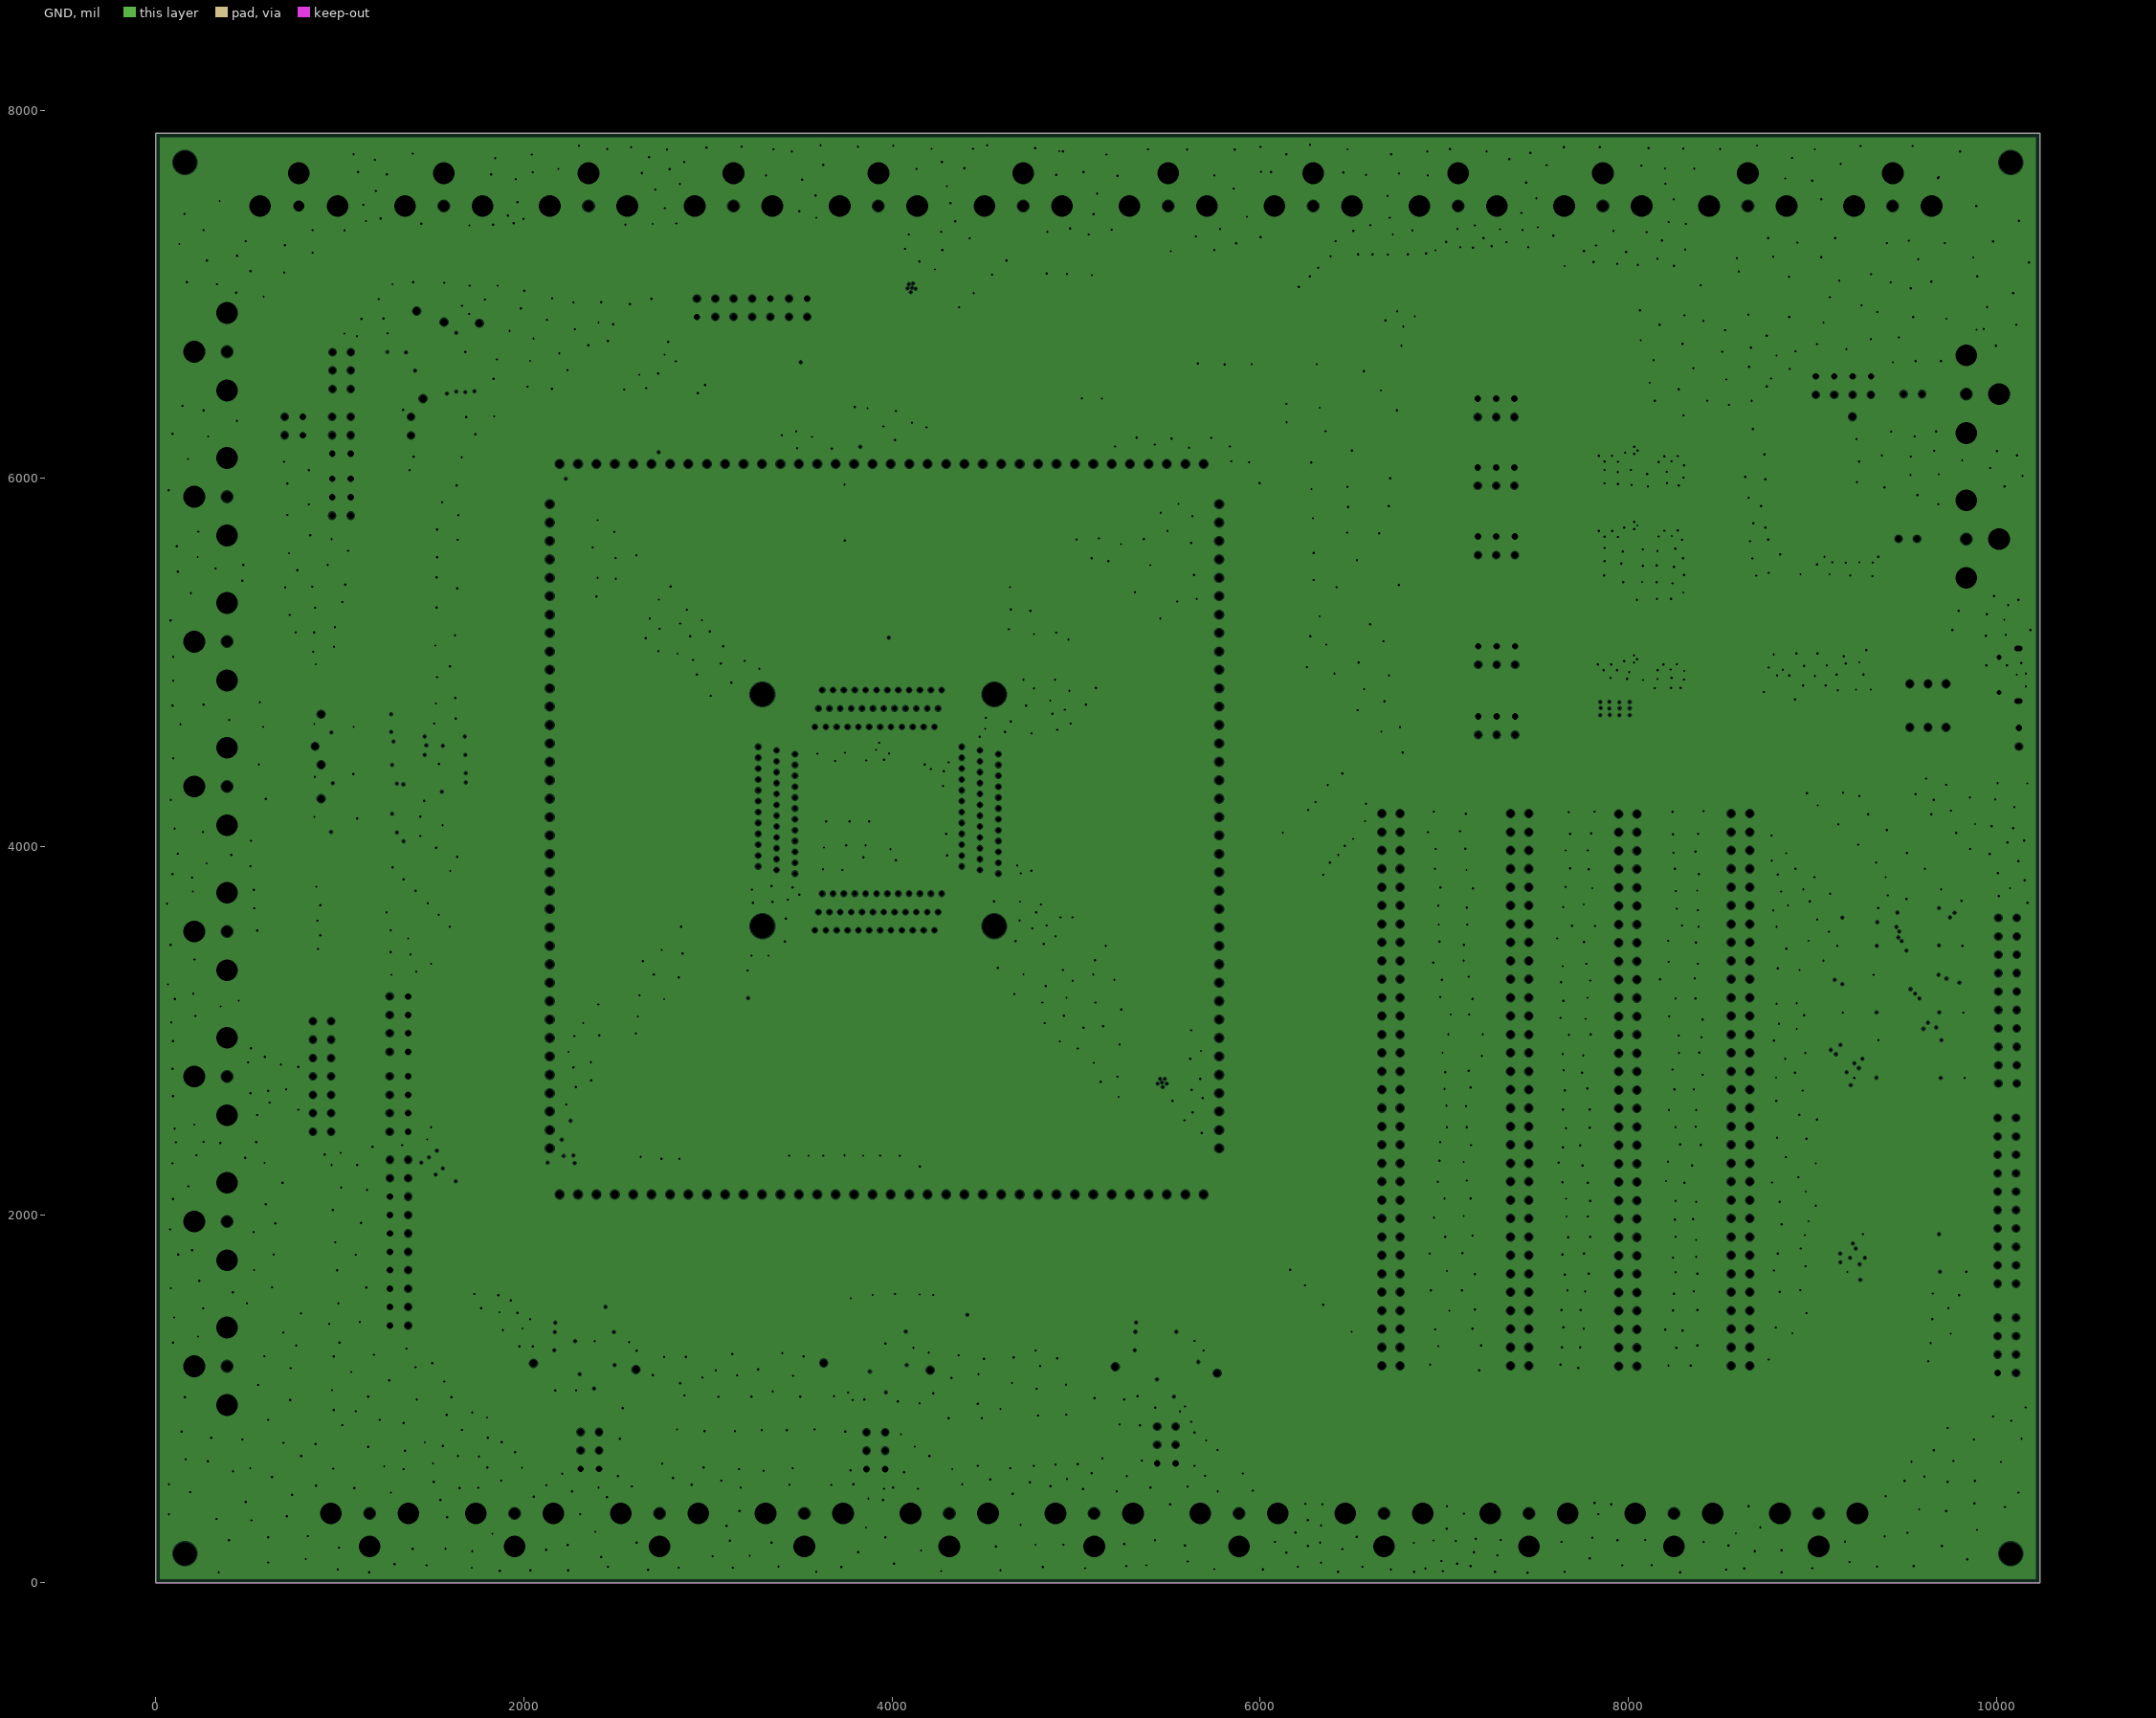
[diagram p0: GND, clearances drawn from the general rule]
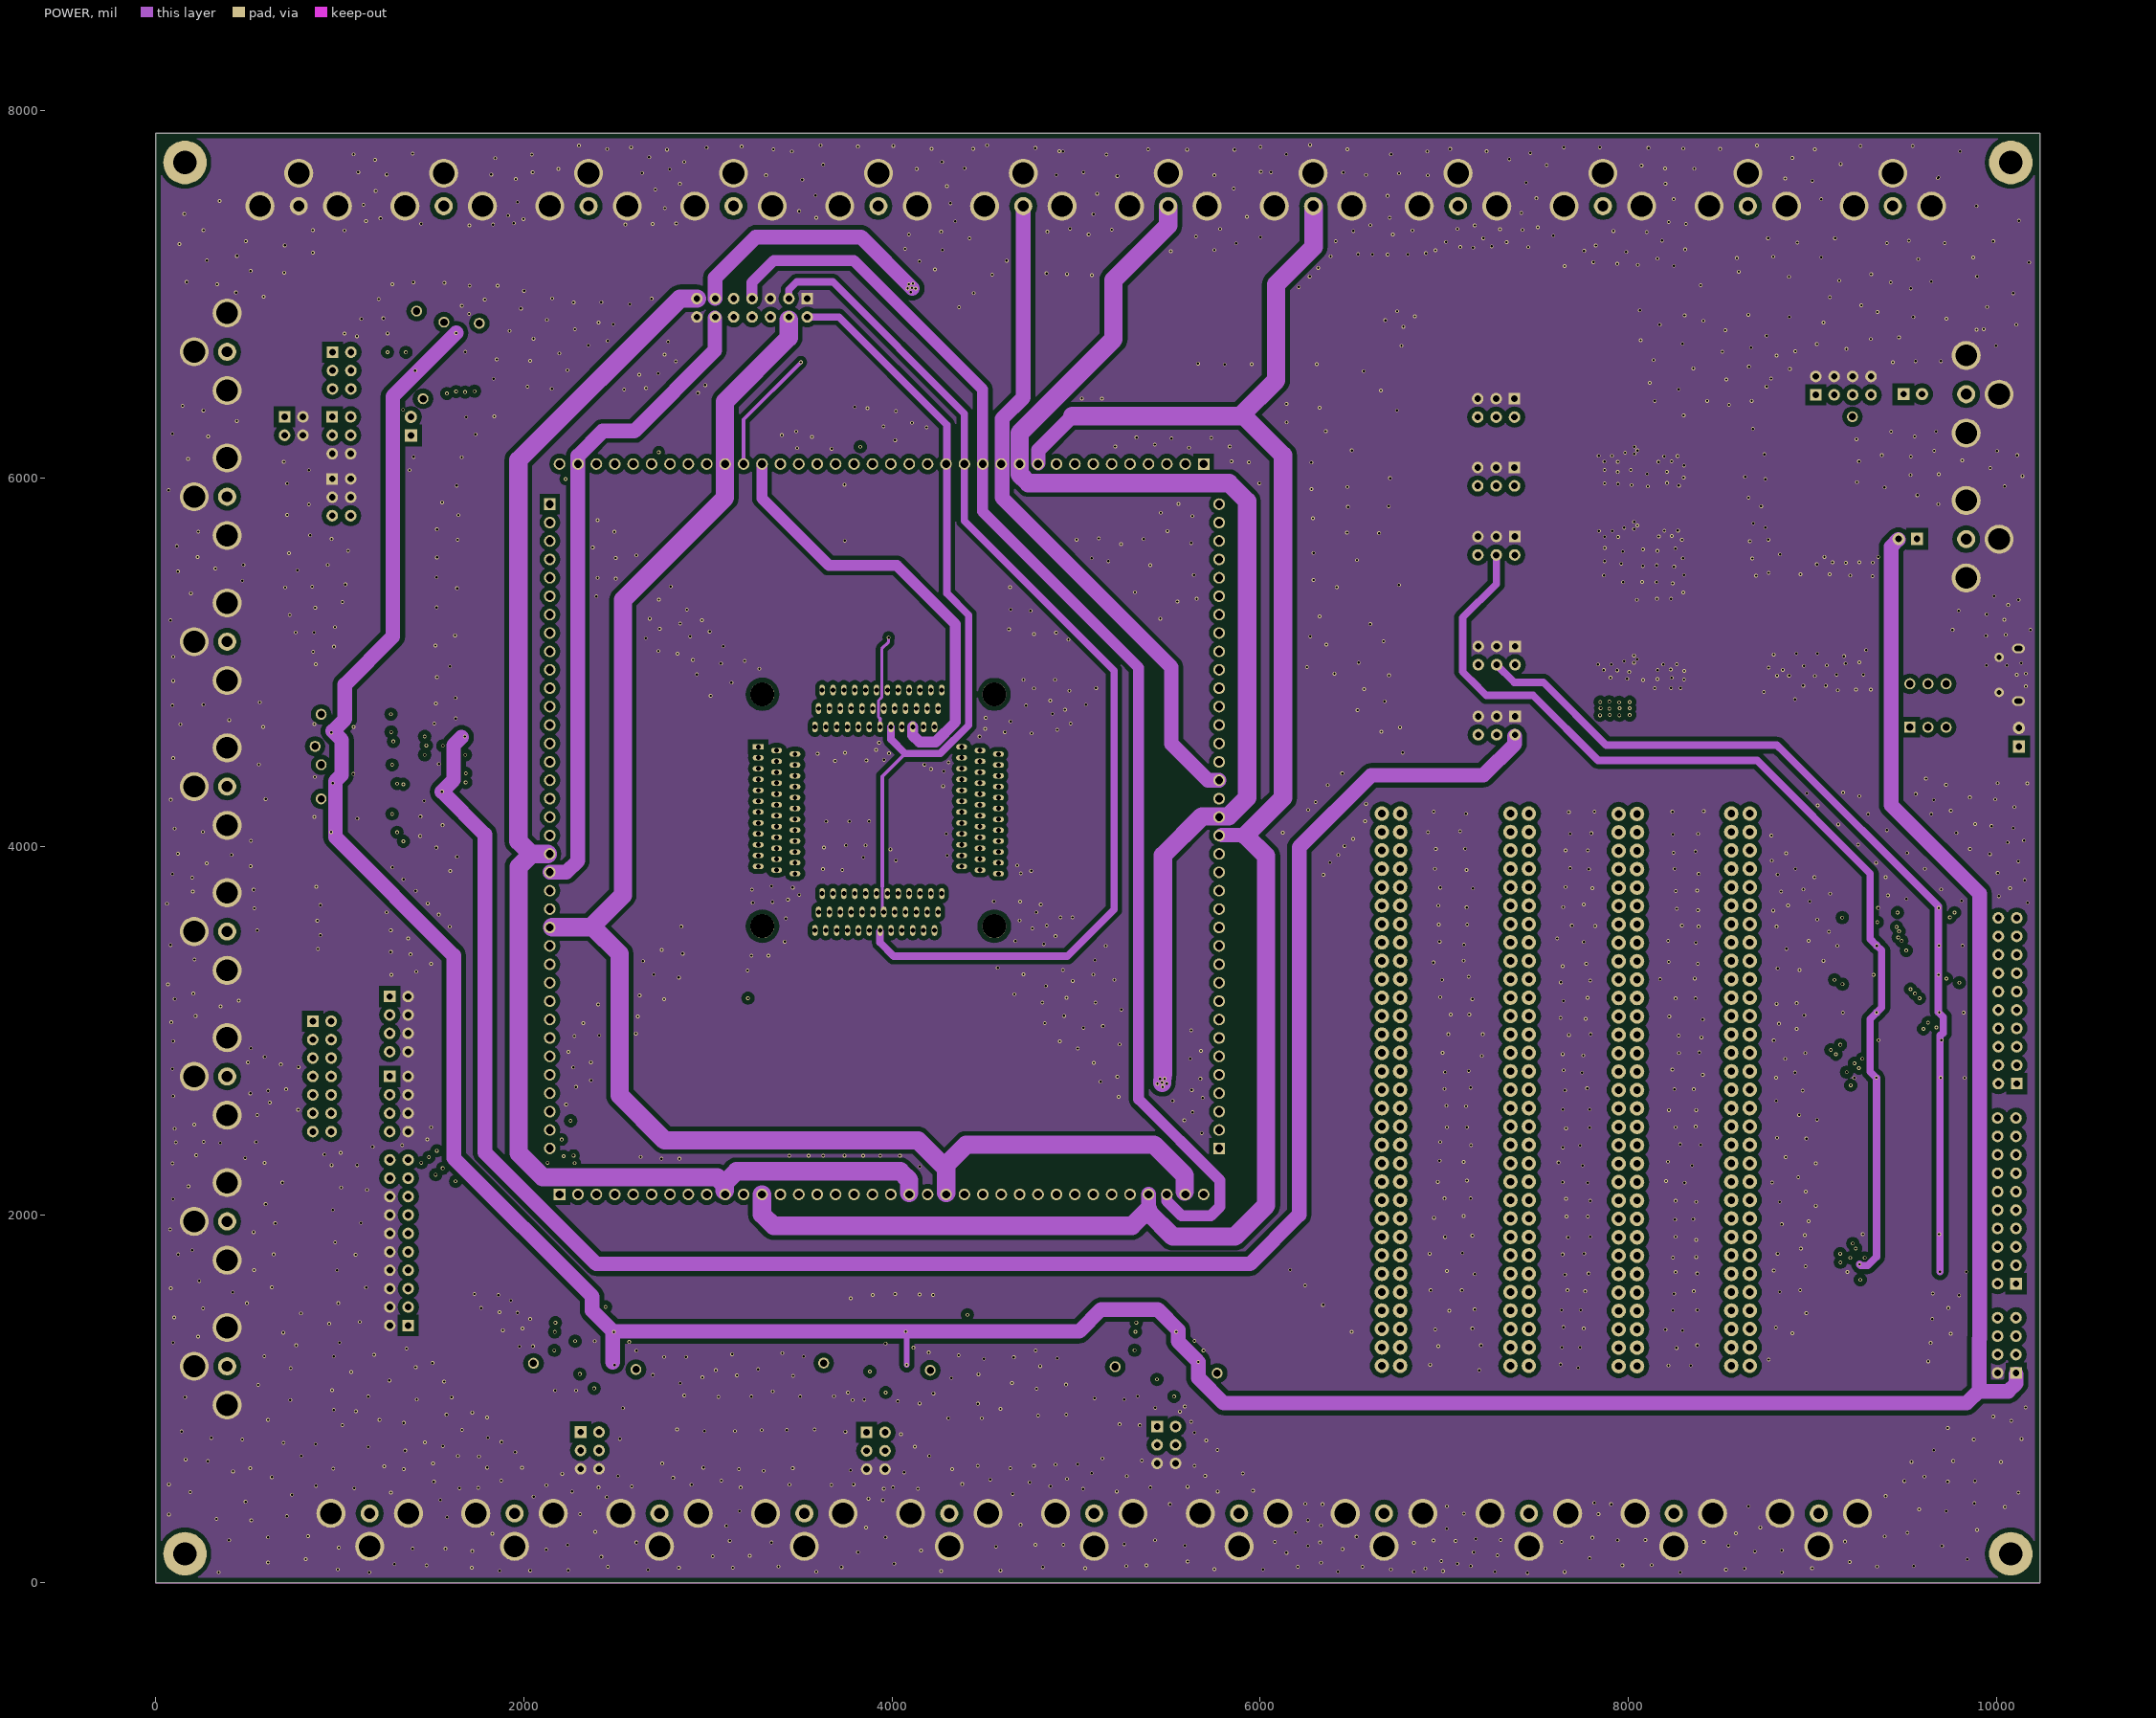
[diagram p1: POWER]
# Altium PCB MISC62794.PcbDoc (part 2 of 7)
## Footprints (in the part's own frame and the unit in brackets; to place one, negate y for a bottom-side part, rotate by r counter-clockwise, add the part's x,y. Pads: shape width x height; smd on the part's side, far side on the other; paste and mask are expansions set on the pad) (continued)
HDR2.54-LI-2x10P [mm] "双排排针，10x2脚"
  rect 1.6x1.6 hole 0.9: 1(-11.43,-1.27)
  round 1.6 hole 0.9: 2(-11.43,1.27) 3(-8.89,-1.27) 4(-8.89,1.27) 5(-6.35,-1.27) 6(-6.35,1.27) 7(-3.81,-1.27) 8(-3.81,1.27) 9(-1.27,-1.27) 10(-1.27,1.27) 11(1.27,-1.27) 12(1.27,1.27) 13(3.81,-1.27) 14(3.81,1.27) 15(6.35,-1.27) 16(6.35,1.27) 17(8.89,-1.27) 18(8.89,1.27) 19(11.43,-1.27) 20(11.43,1.27)
  silkscreen extent -12.7,-2.54 12.7,2.54, body extent -12.7,-2.54 12.7,2.54, height 8.5
HDR2.54-LI-2x31P [mm]
  round 2 hole 1.02: 1(-38.1,1.27) 2(-38.1,-1.27) 3(-35.56,1.27) 4(-35.56,-1.27) 5(-33.02,1.27) 6(-33.02,-1.27) 7(-30.48,1.27) 8(-30.48,-1.27) 9(-27.94,1.27) 10(-27.94,-1.27) 11(-25.4,1.27) 12(-25.4,-1.27) 13(-22.86,1.27) 14(-22.86,-1.27) 15(-20.32,1.27) 16(-20.32,-1.27) 17(-17.78,1.27) 18(-17.78,-1.27) 19(-15.24,1.27) 20(-15.24,-1.27) 21(-12.7,1.27) 22(-12.7,-1.27) 23(-10.16,1.27) 24(-10.16,-1.27) 25(-7.62,1.27) 26(-7.62,-1.27) 27(-5.08,1.27) 28(-5.08,-1.27) 29(-2.54,1.27) 30(-2.54,-1.27) 31(0,1.27) 32(0,-1.27) 33(2.54,1.27) 34(2.54,-1.27) 35(5.08,1.27) 36(5.08,-1.27) 37(7.62,1.27) 38(7.62,-1.27) 39(10.16,1.27) 40(10.16,-1.27) 41(12.7,1.27) 42(12.7,-1.27) 43(15.24,1.27) 44(15.24,-1.27) 45(17.78,1.27) 46(17.78,-1.27) 47(20.32,1.27) 48(20.32,-1.27) 49(22.86,1.27) 50(22.86,-1.27) 51(25.4,1.27) 52(25.4,-1.27) 53(27.94,1.27) 54(27.94,-1.27) 55(30.48,1.27) 56(30.48,-1.27) 57(33.02,1.27) 58(33.02,-1.27) 59(35.56,1.27) 60(35.56,-1.27) 61(38.1,1.27) 62(38.1,-1.27)
  silkscreen extent -39.4,-2.5 39.4,2.5
LED0805-R-RD [mm]
  rect 1x1.4 smd: 1(1.05,0) 2(-1.05,0)
  silkscreen extent -2.22,-1.04 1.99,1.01
M3 [mm]
  round 6 hole 3.2: 1(0,0)
MICRO-USB-SMD_MICROXNJ [mm]
  rect 0.4x1.6 smd paste-100 mask+0.051: 1(-1.3,2.619) 2(-0.65,2.619) 3(0,2.619) 4(0.65,2.619) 5(1.3,2.619)
  round 1.3 hole 0.7 paste+0 mask+0.051: 6(2.425,2.096) 9(-2.425,2.096)
  oval 1.3x1.8 hole 0.7 slot 1.1 at 90 deg paste+0 mask+0.051: 7(3.625,-0.574) 8(-3.625,-0.574)
  silkscreen extent -3.87,-3.22 3.93,2.73
SMB [mil]
  rect 80.61x88.23 smd: 1(-102.02,0) 2(102.02,0)
  silkscreen extent -105,-75 108,75
SO-8 [mm]
  oval 1.865x0.63 smd: 1(-2.682,1.905) 2(-2.682,0.635) 3(-2.682,-0.635) 4(-2.682,-1.905) 5(2.682,-1.905) 6(2.682,-0.635) 7(2.682,0.635) 8(2.682,1.905)
  silkscreen extent -2.83,-2.58 1.52,2.82
SOIC-16_L9.9-W3.9-P1.27-LS6.0-BL [mil]
  oval 23.7x77.6 smd paste+0 mask+2: 1(-169.99,-107.7) 2(-119.99,-107.7) 3(-69.99,-107.7) 4(-19.99,-107.7) 5(30.01,-107.7) 6(80.01,-107.7) 7(130.01,-107.7) 8(180.01,-107.7) 9(180.01,107.7) 10(130.01,107.7) 11(80.01,107.7) 12(30.01,107.7) 13(-19.99,107.7) 14(-69.99,107.7) 15(-119.99,107.7) 16(-169.99,107.7)
  silkscreen extent -206,-111 203,60
SW-TH_6P-L8.0-W8.0-P2.50 [mil]
  rect 60x60 hole 39.37 paste+0 mask+2: 1(-98.43,-118.11)
  round 60 hole 39.37 paste+0 mask+2: 2(0,-118.11) 3(98.42,-118.11) 4(-98.43,118.11) 5(0,118.11) 6(98.42,118.11)
  silkscreen extent -157,-157 157,157
TP1.0 [mm]
  round 1.5 hole 1: 1(0,0)
TSSOP-20_L6.5-W4.4-P0.65-LS6.4-BL [mil]
  oval 68.58x14.33 smd: 1(-113.03,115.16) 2(-113.03,89.57) 3(-113.03,63.98) 4(-113.03,38.39) 5(-113.03,12.79) 6(-113.03,-12.8) 7(-113.03,-38.39) 8(-113.03,-63.98) 9(-113.03,-89.57) 10(-113.03,-115.16) 11(113.03,-115.16) 12(113.03,-89.57) 13(113.03,-63.98) 14(113.03,-38.39) 15(113.03,-12.8) 16(113.03,12.79) 17(113.03,38.39) 18(113.03,63.98) 19(113.03,89.57) 20(113.03,115.16)
  silkscreen extent -119,-131 70,146
WSON-6_L2.0-W2.0-P0.65-BL-EP [mm]
  rect 0.4x0.45 smd paste+0 mask+0.051: 1(-0.65,-0.888) 2(0,-0.888) 3(0.65,-0.888) 4(0.65,1.062) 5(0,1.062) 6(-0.65,1.062)
  rect 1.6x1 smd paste+0 mask+0.051: 7(0,0.087)
  silkscreen extent -1.1,-1.27 1.05,1.14
YAMAICHI_IC51-1444-1354-7 [mm]
  rect 1.5x0.73 hole 0.65: 1(-16.58,8.75)
  oval 1.5x0.73 hole 0.65: 2(-14.04,8.25) 3(-11.5,7.75) 4(-16.58,7.25) 5(-14.04,6.75) 6(-11.5,6.25) 7(-16.58,5.75) 8(-14.04,5.25) 9(-11.5,4.75) 10(-16.58,4.25) 11(-14.04,3.75) 12(-11.5,3.25) 13(-16.58,2.75) 14(-14.04,2.25) 15(-11.5,1.75) 16(-16.58,1.25) 17(-14.04,0.75) 18(-11.5,0.25) 19(-16.58,-0.25) 20(-14.04,-0.75) 21(-11.5,-1.25) 22(-16.58,-1.75) 23(-14.04,-2.25) 24(-11.5,-2.75) 25(-16.58,-3.25) 26(-14.04,-3.75) 27(-11.5,-4.25) 28(-16.58,-4.75) 29(-14.04,-5.25) 30(-11.5,-5.75) 31(-16.58,-6.25) 32(-14.04,-6.75) 33(-11.5,-7.25) 34(-16.58,-7.75) 35(-14.04,-8.25) 36(-11.5,-8.75) 73(16.58,-8.75) 74(14.04,-8.25) 75(11.5,-7.75) 76(16.58,-7.25) 77(14.04,-6.75) 78(11.5,-6.25) 79(16.58,-5.75) 80(14.04,-5.25) 81(11.5,-4.75) 82(16.58,-4.25) 83(14.04,-3.75) 84(11.5,-3.25) 85(16.58,-2.75) 86(14.04,-2.25) 87(11.5,-1.75) 88(16.58,-1.25) 89(14.04,-0.75) 90(11.5,-0.25) 91(16.58,0.25) 92(14.04,0.75) 93(11.5,1.25) 94(16.58,1.75) 95(14.04,2.25) 96(11.5,2.75) 97(16.58,3.25) 98(14.04,3.75) 99(11.5,4.25) 100(16.58,4.75) 101(14.04,5.25) 102(11.5,5.75) 103(16.58,6.25) 104(14.04,6.75) 105(11.5,7.25) 106(16.58,7.75) 107(14.04,8.25) 108(11.5,8.75)
  oval 0.73x1.5 hole 0.65: 37(-8.75,-16.58) 38(-8.25,-14.04) 39(-7.75,-11.5) 40(-7.25,-16.58) 41(-6.75,-14.04) 42(-6.25,-11.5) 43(-5.75,-16.58) 44(-5.25,-14.04) 45(-4.75,-11.5) 46(-4.25,-16.58) 47(-3.75,-14.04) 48(-3.25,-11.5) 49(-2.75,-16.58) 50(-2.25,-14.04) 51(-1.75,-11.5) 52(-1.25,-16.58) 53(-0.75,-14.04) 54(-0.25,-11.5) 55(0.25,-16.58) 56(0.75,-14.04) 57(1.25,-11.5) 58(1.75,-16.58) 59(2.25,-14.04) 60(2.75,-11.5) 61(3.25,-16.58) 62(3.75,-14.04) 63(4.25,-11.5) 64(4.75,-16.58) 65(5.25,-14.04) 66(5.75,-11.5) 67(6.25,-16.58) 68(6.75,-14.04) 69(7.25,-11.5) 70(7.75,-16.58) 71(8.25,-14.04) 72(8.75,-11.5) 109(8.75,16.58) 110(8.25,14.04) 111(7.75,11.5) 112(7.25,16.58) 113(6.75,14.04) 114(6.25,11.5) 115(5.75,16.58) 116(5.25,14.04) 117(4.75,11.5) 118(4.25,16.58) 119(3.75,14.04) 120(3.25,11.5) 121(2.75,16.58) 122(2.25,14.04) 123(1.75,11.5) 124(1.25,16.58) 125(0.75,14.04) 126(0.25,11.5) 127(-0.25,16.58) 128(-0.75,14.04) 129(-1.25,11.5) 130(-1.75,16.58) 131(-2.25,14.04) 132(-2.75,11.5) 133(-3.25,16.58) 134(-3.75,14.04) 135(-4.25,11.5) 136(-4.75,16.58) 137(-5.25,14.04) 138(-5.75,11.5) 139(-6.25,16.58) 140(-6.75,14.04) 141(-7.25,11.5) 142(-7.75,16.58) 143(-8.25,14.04) 144(-8.75,11.5)
  round 3.3 hole 3.3 unplated: ""(-16,-16) ""(-16,16) ""(16,-16) ""(16,16)
  silkscreen extent -24.51,-23.98 23.5,25

## Part data
C1 C2 C3 C4 C5 C6 C7 C8 C9 C10 C11 C20 C21 C22 C23 C24 C25 C26 C27 C28 C30 C31 C32 C33 C34 C35 C36 C37 C38 C39 C40 C41: library part CAP, "capacitor model"
D1: "diode"
IC1 U1 U2 U3 U4 U5 U6 U7 U8 U9 U10 U11: "IC"
IC2 IC3 IC4: "LDO"
JP1 JP2 JP3 JP4 JP5 JP6 JP7 JP8 JP11 JP12 JP13 JP14 JP16 JP17 JP20 JP30 JP31 JP32 JP33 JP34 JP35 JP36 JP37 JP38 JP39 JP43 JP44 JP45 JP46: "pin header"
JP40 JP41 JP42: library part "HEADER 36X1", "pin header"
LED_BLUE: "light-emitting diode"
R1 R2 R3 R4 R5 R6 R7 R8 R9 R10 R11 R12 R13 R14 R15 R16 R20: library part RES, "resistor model"
S1: library part switch6, "six-pin self-locking switch"
SOCKET1: library part M189_4K, "array"
SP1 SP2 SP3 SP4: "M3 interface"
TP1 TP2 TP3 TP4 TP5 TP6 TP7 TP8 TP9 TP10 TP11 TP12 TP13 TP14 TP15: library part TP, "TP"

## Via types
v1: diameter 20, hole 12, Top Layer to Bottom Layer, 1759 vias

## Nets (pads, with @x,y where several pads share a name; then routed paths per layer and width w, separated by ;. In a path a pad name is that pad's centre, name@x,y a point inside that pad or via, vN(x,y) a via of type N, cw(c..) or ccw(c..) an arc to the next point about the centre after c; other vN are vias at no path point)
3V3: C31.1 C33.1 C35.1 C37.1 C40.1 C41.1 IC4.1 JP45.4 JP45.6 JP46.4 JP46.6 U12.2 U12.10 U13.2 U13.10 U14.2 U14.10 U15.2 U15.10 | length 5547
  Top Layer w16: U14.2@9635.03,3461.44 C35.1@9725.01,3461.44 ; U14.10@9635.03,3666.17 v1(9687.83,3666.17) ; U15.2@9636.03,1689.44 v1@9694,1689.44 ; U15.10@9636.03,1894.17 v1(9689.17,1894.17) ; U13.2@9637.03,3098.44 C33.1@9725.01,3098.44 ; U13.10@9637.03,3303.17 v1(9686.17,3303.17) ; U12.2@9638.03,2743.44 v1(9697.56,2743.44) ; U12.10@9638.03,2948.17 v1(9702.17,2948.17) ; v1(9694,1690) v1@9694,1689.44 ; v1@9699,2743.44 C31.1@9734.01,2743.44 ; C37.1@9742.56,1689.44 v1@9694,1689.44
  POWER w40: JP46.4@7285,4987.46 7380.46,4892 7539,4892 7880,4551 8808,4551 8846,4513 ; 8846.5,4513.5 9685,3675 9685,3100 9712,3073 9712,2987 9711,2986 ; v1(9694,1690) 9694,2973 9709,2988
  other v1: 9690,3099 9689,3462
CSB_ADD<0>: JP42.4 SOCKET1.110 U12.20 | length 8790.6
  Top Layer w6: SOCKET1.110@4249.8,4749.77 4328,4827.97 4328,4911 4478,5061 4478,5492 4809,5823 5136,5823 JP42.4@5377,6064 ; v1@9216,2708 9224,2716 9225.85,2717.85 9234.41,2717.85 9235.96,2716.29 9410.41,2716.29 U12.20@9411.97,2717.85
  Bottom Layer w6: SOCKET1.110@4249.8,4749.77 4469.03,4969 5185,4969 5536,4618 6329,4618 6655,4292 8692,4292 9209,3775 v1(9209,2703)
CSB_ADD<0>_MCU: JP43.1 U12.1 | length 504.2
  Top Layer w6: U12.1@9638.03,2717.85 9681.15,2717.85 9713,2686 9926,2686 9959,2653 10056,2653 JP43.1@10098,2695
CSB_ADD<1>: JP42.2 SOCKET1.111 U12.18 | length 9062.1
  Top Layer w6: SOCKET1.111@4230.12,4649.77 4241.77,4649.77 4375,4783 4375,4893 4538,5056 4538,5471 4822,5755 5270,5755 JP42.2@5589,6074 ; v1@9190,2777 9341,2777 9348.97,2769.03 U12.18@9411.97,2769.03
  Bottom Layer w6: SOCKET1.111@4230.12,4649.77 4295,4714.65 4295,4751 4495,4951 5154,4951 5502,4603 6293,4603 6632,4264 8680,4264 9187,3757 v1(9187,2774)
CSB_ADD<1>_MCU: JP43.2 U12.3 | length 382
  Top Layer w6: U12.3@9638.03,2769.03 9703.03,2769.03 9712,2778 9930,2778 JP43.2@9991,2717
CSB_ADD<2>: JP42.7 SOCKET1.112 U12.17 | length 8464.4
  Top Layer w6: SOCKET1.112@4210.43,4849.77 4210.43,4900.43 4368,5058 4368,5519 4760,5911 4928,5911 JP42.7@5080,6063 ; v1@9258.38,2794.62 U12.17@9411.97,2794.62
  Bottom Layer w6: SOCKET1.112@4210.43,4849.77 4210.43,4883.43 4259,4932 4341,4932 4433,5024 5229,5024 5534,4719 6317,4719 6690,4346 8696,4346 9253,3789 v1(9253,2796)
CSB_ADD<2>_MCU: JP43.3 U12.4 | length 485.4
  Top Layer w6: U12.4@9638.03,2794.62 9952.38,2794.62 9981,2766 10072,2766 JP43.3@10100,2794
CSB_ADD<3>: JP42.5 SOCKET1.113 U12.16 | length 8804.6
  Top Layer w6: SOCKET1.113@4190.75,4749.77 4195,4754.02 4195,4768 4209,4782 4231,4782 4253,4804 4283,4804 4310,4831 4310,4924 4450,5064 4450,5508 4793,5851 5071,5851 JP42.5@5290,6070 ; v1@9226.78,2820.22 U12.16@9411.97,2820.22
  Bottom Layer w6: SOCKET1.113@4190.75,4749.77 4237,4796.02 4237,4870 4273,4906 4360,4906 4455,5001 5205,5001 5502,4704 6286,4704 6676,4314 8697,4314 9229,3782 v1(9229,2822)
CSB_ADD<3>_MCU: JP43.4 U12.5 | length 362.8
  Top Layer w6: U12.5@9638.03,2820.22 JP43.4@10000.78,2820.22
CSB_ADD<4>: JP42.3 SOCKET1.114 U12.15 | length 9221.2
  Top Layer w6: SOCKET1.114@4171.06,4649.77 4220.29,4699 4260,4699 4348,4787 4348,4897 4507,5056 4507,5479 4821.5,5793.5 5206.5,5793.5 JP42.3@5479,6066 ; v1@9272.81,2845.81 U12.15@9411.97,2845.81
  Bottom Layer w6: SOCKET1.114@4171.06,4649.77 4171.06,4686.94 4162,4696 4162,4787 4184,4809 4184,4890 4247,4953 4336,4953 4425,5042 5237,5042 5477,4802 6271,4802 6703,4370 8707,4370 9274,3803 v1@9274,2847
  other v1: 9272,2847
CSB_ADD<4>_MCU: JP43.5 U12.6 | length 490.7
  Top Layer w6: U12.6@9638.03,2845.81 9816.81,2845.81 9840,2869 10071,2869 JP43.5@10105,2903
DAC1: JP3.1 R1.2 TP1.1 U8.1 | length 630.4
  Top Layer w20: TP1.1@5208,1161 5207,1160 5207,978 5274,911 5378.2,911 JP3.1@5440.19,849.02 ; TP1.1@5227,1173 5304,1173 5313.33,1163.67 U8.1@5383.51,1163.67
DAC2: JP3.2 R3.1 TP2.1 U8.7 | length 483.7
  Top Layer w20: JP3.2@5535,864 5494,905 5494,1041 5567,1114 U8.7@5591,1114 ; U8.7@5591,1113.67 U8.7@5594.73,1113.67 5638.67,1113.67 5664,1139 TP2.1@5743,1139
DAC3: JP4.1 R5.2 TP3.1 U10.1 | length 718.7
  Top Layer w20: TP3.1@3630,1186 3612,1168 3612,957 3666,903 3775.86,903 JP4.1@3861.48,817.38 ; TP3.1@3639,1192 3724,1192 3732.33,1183.67 U10.1@3810.51,1183.67
DAC4: JP4.2 R7.1 TP4.1 U10.7 | length 573.3
  Top Layer w20: JP4.2@3954,833 3929,858 3929,1076 3986.67,1133.67 U10.7@4021.73,1133.67 4090.67,1133.67 4111,1154 TP4.1@4201,1154 ; JP4.2@3961.48,817.38 JP4.2@3961.48,833
DAC5: JP5.1 R9.2 TP5.1 U9.1 | length 670
  Top Layer w20: TP5.1@2049,1174 2049,1001 2103,947 2179.2,947 JP5.1@2307.19,819.02 ; TP5.1@2068,1192 R9.2@2137,1192 ; R9.2@2134.12,1193.33 2190.67,1193.33 U9.1@2198,1186 ; U9.1@2198,1182.67 U9.1@2225.51,1182.67